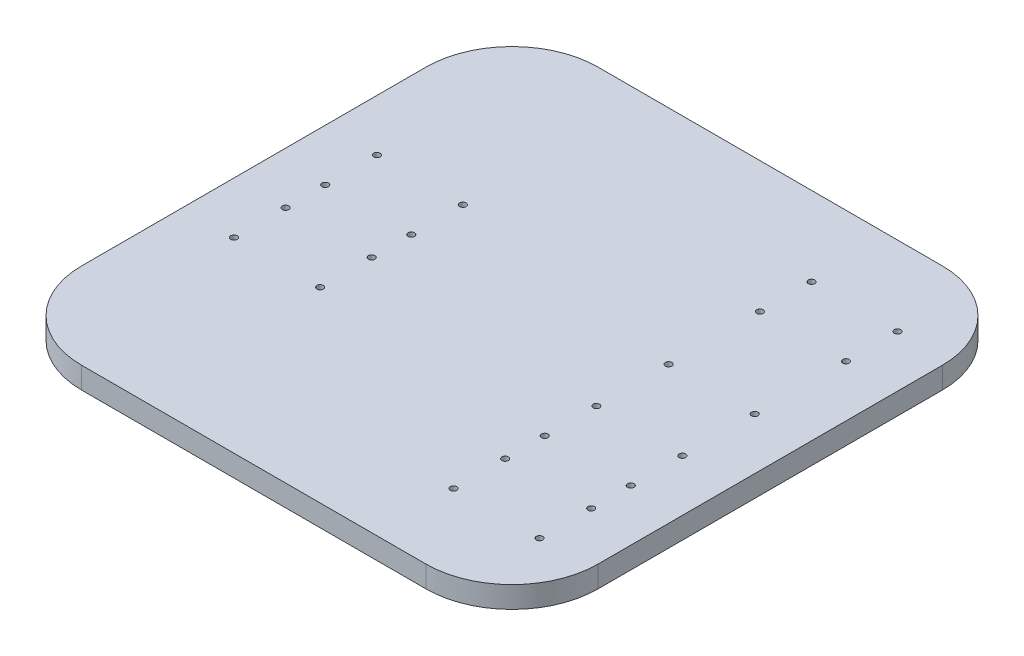
from build123d import *

# Parameters (mm, degrees)
BOSS_EXTRUDE1_DEPTH = 5
SKETCH4_R           = 0.75
CUT_EXTRUDE1_DEPTH  = 86


with BuildPart() as part:
    # Sketch1 → Boss-Extrude1 (new body)
    with BuildSketch(Plane(origin=(0, 0, 0), x_dir=(1, 0, 0), z_dir=(0, 1, 0))):
        with BuildLine():
            Line((-40, -60), (40, -60))
            ThreePointArc((40, -60), (54.142135624, -54.142135624), (60, -40))
            Line((60, -40), (60, 40))
            ThreePointArc((60, 40), (54.142135624, 54.142135624), (40, 60))
            Line((40, 60), (-40, 60))
            ThreePointArc((-40, 60), (-54.142135624, 54.142135624), (-60, 40))
            Line((-60, 40), (-60, -40))
            ThreePointArc((-60, -40), (-54.142135624, -54.142135624), (-40, -60))
        make_face()
    extrude(amount=BOSS_EXTRUDE1_DEPTH)

    # Sketch4 → Cut-Extrude1 (cut, through all)
    with BuildSketch(Plane(origin=(0, 5, 0), x_dir=(1, 0, 0), z_dir=(0, 1, 0))):
        with Locations(Location((-48, 16.6, 0), (0, 0, 270))):
            Circle(SKETCH4_R)
        with Locations(Location((-28, 16.6, 0), (0, 0, 90))):
            Circle(SKETCH4_R)
        with Locations(Location((-48, 4.6, 0), (0, 0, 90))):
            Circle(SKETCH4_R)
        with Locations(Location((-28, 4.6, 0), (0, 0, 270))):
            Circle(SKETCH4_R)
        with Locations(Location((-28, -4.6, 0), (0, 0, 90))):
            Circle(SKETCH4_R)
        with Locations(Location((-48, -4.6, 0), (0, 0, 270))):
            Circle(SKETCH4_R)
        with Locations(Location((-28, -16.6, 0), (0, 0, 270))):
            Circle(SKETCH4_R)
        with Locations(Location((-48, -16.6, 0), (0, 0, 90))):
            Circle(SKETCH4_R)
        with Locations(Location((28, 41.6, 0), (0, 0, 270))):
            Circle(SKETCH4_R)
        with Locations(Location((48, 41.6, 0), (0, 0, 90))):
            Circle(SKETCH4_R)
        with Locations(Location((28, 29.6, 0), (0, 0, 90))):
            Circle(SKETCH4_R)
        with Locations(Location((48, 29.6, 0), (0, 0, 270))):
            Circle(SKETCH4_R)
        with Locations(Location((48, 8.4, 0), (0, 0, 270))):
            Circle(SKETCH4_R)
        with Locations(Location((28, 8.4, 0), (0, 0, 90))):
            Circle(SKETCH4_R)
        with Locations(Location((28, -8.4, 0), (0, 0, 270))):
            Circle(SKETCH4_R)
        with Locations(Location((48, -8.4, 0), (0, 0, 90))):
            Circle(SKETCH4_R)
        with Locations(Location((28, -20.4, 0), (0, 0, 90))):
            Circle(SKETCH4_R)
        with Locations(Location((48, -20.4, 0), (0, 0, 270))):
            Circle(SKETCH4_R)
        with Locations(Location((48, -29.6, 0), (0, 0, 90))):
            Circle(SKETCH4_R)
        with Locations(Location((28, -29.6, 0), (0, 0, 270))):
            Circle(SKETCH4_R)
        with Locations(Location((48, -41.6, 0), (0, 0, 270))):
            Circle(SKETCH4_R)
        with Locations(Location((28, -41.6, 0), (0, 0, 90))):
            Circle(SKETCH4_R)
    extrude(amount=-CUT_EXTRUDE1_DEPTH, mode=Mode.SUBTRACT)


solid = part.part
